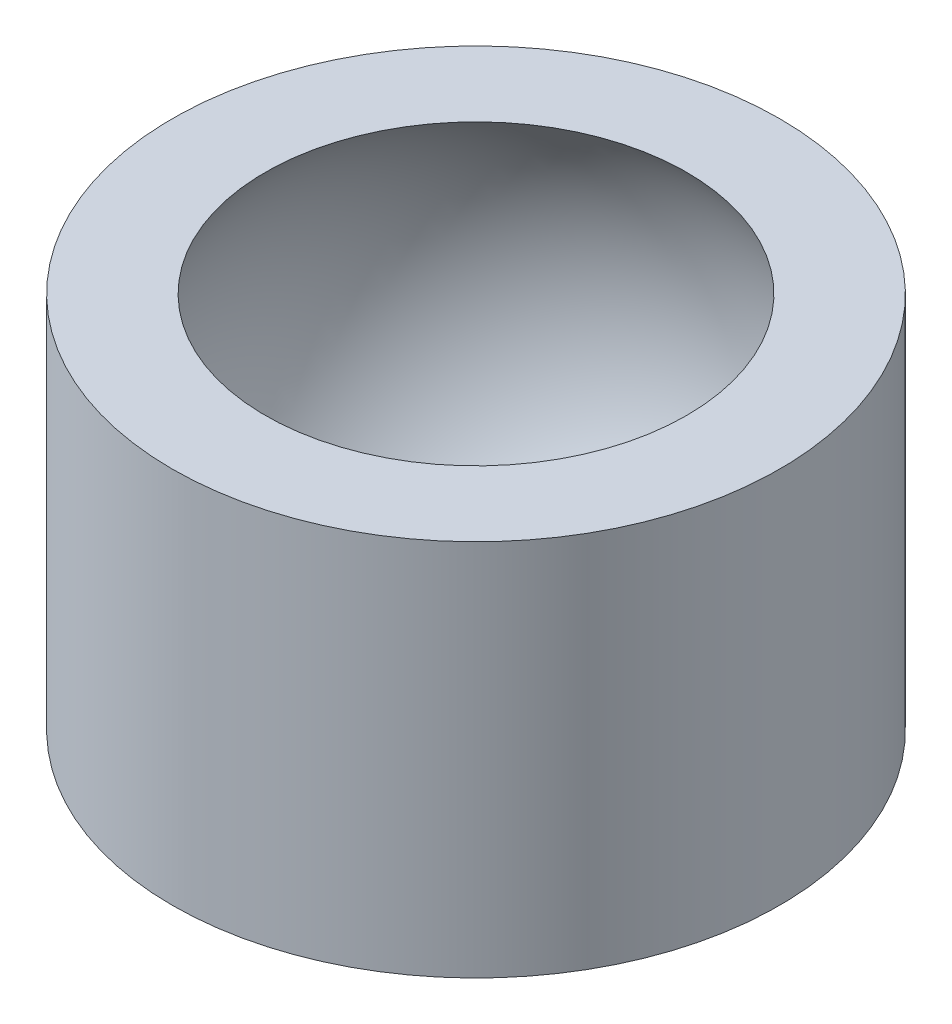
from build123d import *


with BuildPart() as part:
    # 草图1 → 旋转1 (revolve)
    with BuildSketch(Plane.XY):
        with BuildLine():
            Line((15.612494996, 12.5), (22.5, 12.5))
            Line((22.5, 12.5), (22.5, -15.5))
            Line((22.5, -15.5), (19.3, -15.5))
            Line((19.3, -15.5), (15.612494996, -12.5))
            ThreePointArc((15.612494996, -12.5), (20, 0), (15.612494996, 12.5))
        make_face()
    revolve(axis=Axis((0, 29.923042414, 0), (0, -1, 0)))


solid = part.part
